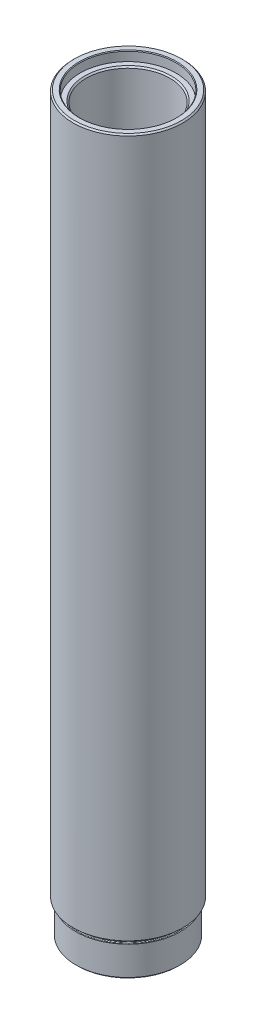
from build123d import *

# Parameters (mm, degrees)
SKETCH1_R                  = 40
SKETCH1_R_2                = 30
BOSS_EXTRUDE1_DEPTH        = 537.5
CUT_EXTRUDE1_START         = -25
SKETCH2_R                  = 55.029082457
SKETCH2_R_2                = 36.75
CUT_EXTRUDE1_DEPTH         = 3
SKETCH3_R                  = 40
SKETCH3_R_2                = 38
CUT_EXTRUDE2_DEPTH         = 25
CHAMFER1_SIZE              = 1
SKETCH4_R                  = 33.575067705
BOSS_EXTRUDE2_DEPTH        = 40
SKETCH5_R                  = 25
CUT_EXTRUDE3_DEPTH         = 6
SKETCH6_R                  = 21.5
CUT_EXTRUDE4_DEPTH         = 535.501870904
CHAMFER2_SIZE              = 1
SKETCH9_R                  = 30
CUT_EXTRUDE7_DEPTH         = 40
SKETCH10_R                 = 35
CUT_EXTRUDE8_DEPTH         = 7
M64X4_0_TAPPED_HOLE1_D     = 60
M64X4_0_TAPPED_HOLE1_DEPTH = 20
M64X4_0_TAPPED_HOLE1_TIP   = 18.025818571
CHAMFER3_SIZE              = 0.5
CHAMFER4_SIZE              = 0.5
SKETCH13_R                 = 40
CUT_EXTRUDE9_DEPTH         = 3
CHAMFER5_SIZE              = 1
CHAMFER7_SIZE              = 0.5
FILLET1_R                  = 0.5
M64X3_0_TAPPED_HOLE1_D     = 61
M64X3_0_TAPPED_HOLE1_DEPTH = 55
M64X3_0_TAPPED_HOLE1_TIP   = 18.32624888
CHAMFER8_SIZE              = 1


with BuildPart() as part:
    # Sketch1 → Boss-Extrude1 (new body)
    with BuildSketch(Plane(origin=(0, 0, 0), x_dir=(1, 0, 0), z_dir=(0, 1, 0))):
        with Locations(Location((0, 0, 0), (0, 0, 270))):
            Circle(SKETCH1_R)
        with Locations(Location((0, 0, 0), (0, 0, 270))):
            Circle(SKETCH1_R_2, mode=Mode.SUBTRACT)
    extrude(amount=BOSS_EXTRUDE1_DEPTH)

    # Sketch2 → Cut-Extrude1 (cut)
    with BuildSketch(Plane.XZ.offset(CUT_EXTRUDE1_START)):
        Circle(SKETCH2_R)
        with Locations(Location((0, 0, 0), (0, 0, 270))):
            Circle(SKETCH2_R_2, mode=Mode.SUBTRACT)
    extrude(amount=-CUT_EXTRUDE1_DEPTH, mode=Mode.SUBTRACT)

    # Sketch3 → Cut-Extrude2 (cut)
    with BuildSketch(Plane.XZ):
        with Locations(Location((0, 0, 0), (0, 0, 270))):
            Circle(SKETCH3_R)
        with Locations(Location((0, 0, 0), (0, 0, 270))):
            Circle(SKETCH3_R_2, mode=Mode.SUBTRACT)
    extrude(amount=-CUT_EXTRUDE2_DEPTH, mode=Mode.SUBTRACT)

    # Chamfer1
    chamfer1_edges = [part.edges().sort_by_distance(p)[0] for p in [
        (0, 0, 38),
        (0, 537.5, -40),
    ]]
    chamfer(chamfer1_edges, length=CHAMFER1_SIZE)

    # Sketch4 → Boss-Extrude2 (add)
    with BuildSketch(Plane(origin=(0, 537.5, 0), x_dir=(1, 0, 0), z_dir=(0, 1, 0))):
        Circle(SKETCH4_R)
    extrude(amount=-BOSS_EXTRUDE2_DEPTH)

    # Sketch5 → Cut-Extrude3 (cut)
    with BuildSketch(Plane(origin=(0, 537.5, 0), x_dir=(1, 0, 0), z_dir=(0, 1, 0))):
        with Locations(Location((0, 0, 0), (0, 0, 270))):
            Circle(SKETCH5_R)
    extrude(amount=-CUT_EXTRUDE3_DEPTH, mode=Mode.SUBTRACT)

    # Sketch6 → Cut-Extrude4 (cut, through all)
    with BuildSketch(Plane(origin=(0, 531.5, 0), x_dir=(1, 0, 0), z_dir=(0, 1, 0))):
        with Locations(Location((0, 0, 0), (0, 0, 270))):
            Circle(SKETCH6_R)
    extrude(amount=-CUT_EXTRUDE4_DEPTH, mode=Mode.SUBTRACT)

    # Chamfer2
    chamfer2_edges = [part.edges().sort_by_distance(p)[0] for p in [
        (0, 531.5, -21.5),
    ]]
    chamfer(chamfer2_edges, length=CHAMFER2_SIZE)

    # Sketch9 → Cut-Extrude7 (cut)
    with BuildSketch(Plane.XZ.offset(-497.5)):
        with Locations(Location((0, 0, 0), (0, 0, 90))):
            Circle(SKETCH9_R)
    extrude(amount=-CUT_EXTRUDE7_DEPTH, mode=Mode.SUBTRACT)

    # Sketch10 → Cut-Extrude8 (cut)
    with BuildSketch(Plane(origin=(0, 537.5, 0), x_dir=(1, 0, 0), z_dir=(0, 1, 0))):
        with Locations(Location((0, 0, 0), (0, 0, 270))):
            Circle(SKETCH10_R)
    extrude(amount=-CUT_EXTRUDE8_DEPTH, mode=Mode.SUBTRACT)

    # M64x4.0 Tapped Hole1
    with Locations(Plane(origin=(0, 530.5, 0), x_dir=(1, 0, 0), z_dir=(0, 1, 0))):
        with Locations((0, 0)):
            Hole(M64X4_0_TAPPED_HOLE1_D / 2, depth=M64X4_0_TAPPED_HOLE1_DEPTH)
            with Locations((0, 0, -(M64X4_0_TAPPED_HOLE1_DEPTH + M64X4_0_TAPPED_HOLE1_TIP / 2))):  # 118° drill point
                Cone(0, M64X4_0_TAPPED_HOLE1_D / 2, M64X4_0_TAPPED_HOLE1_TIP, mode=Mode.SUBTRACT)

    # Chamfer3
    chamfer3_edges = [part.edges().sort_by_distance(p)[0] for p in [
        (0, 537.5, -35),
    ]]
    chamfer(chamfer3_edges, length=CHAMFER3_SIZE)

    # Chamfer4
    chamfer4_edges = [part.edges().sort_by_distance(p)[0] for p in [
        (0, 530.5, -30),
    ]]
    chamfer(chamfer4_edges, length=CHAMFER4_SIZE)

    # Sketch13 → Cut-Extrude9 (cut)
    with BuildSketch(Plane.XZ):
        with Locations(Location((0, 0, 0), (0, 0, 270))):
            Circle(SKETCH13_R)
    extrude(amount=-CUT_EXTRUDE9_DEPTH, mode=Mode.SUBTRACT)

    # Chamfer5
    chamfer5_edges = [part.edges().sort_by_distance(p)[0] for p in [
        (0, 3, 38),
    ]]
    chamfer(chamfer5_edges, length=CHAMFER5_SIZE)

    # Chamfer7
    chamfer7_edges = [part.edges().sort_by_distance(p)[0] for p in [
        (0, 28, -40),
    ]]
    chamfer(chamfer7_edges, length=CHAMFER7_SIZE)

    # Fillet1
    fillet1_edges = [part.edges().sort_by_distance(p)[0] for p in [
        (0, 28, 36.75),
        (0, 25, 36.75),
    ]]
    fillet(fillet1_edges, radius=FILLET1_R)

    # M64x3.0 Tapped Hole1
    with Locations(Plane(origin=(0, 530.5, 0), x_dir=(1, 0, 0), z_dir=(0, 1, 0))):
        with Locations((0, 0)):
            Hole(M64X3_0_TAPPED_HOLE1_D / 2, depth=M64X3_0_TAPPED_HOLE1_DEPTH)
            with Locations((0, 0, -(M64X3_0_TAPPED_HOLE1_DEPTH + M64X3_0_TAPPED_HOLE1_TIP / 2))):  # 118° drill point
                Cone(0, M64X3_0_TAPPED_HOLE1_D / 2, M64X3_0_TAPPED_HOLE1_TIP, mode=Mode.SUBTRACT)

    # Chamfer8
    chamfer8_edges = [part.edges().sort_by_distance(p)[0] for p in [
        (30.5, 530.5, 0),
    ]]
    chamfer(chamfer8_edges, length=CHAMFER8_SIZE)


solid = part.part
